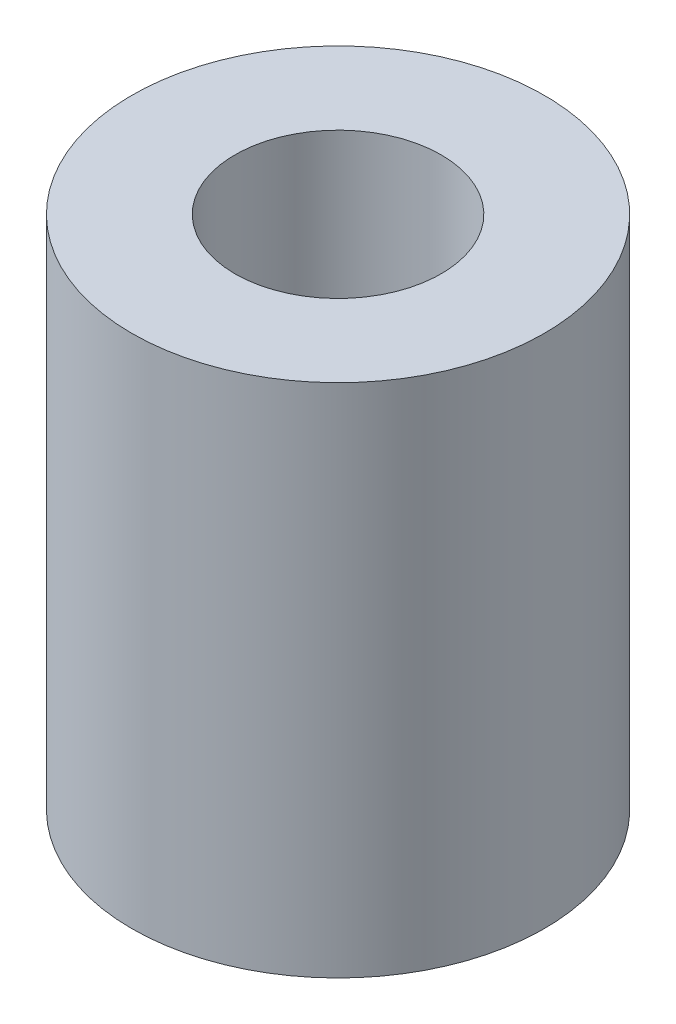
SolidWorks part; units mm, degrees
ref_plane "Front" through (0, 0, 0) normal (0, 0, 1) x (1, 0, 0)
ref_plane "Top" through (0, 0, 0) normal (0, 1, 0) x (1, 0, 0)
ref_plane "Right" through (0, 0, 0) normal (1, 0, 0) x (0, 0, -1)
sketch "Sketch1" plane through (0, 0, 0) normal (0, 1, 0) x (1, 0, 0)
  circle A0 centre (0, 0) radius 20
  circle A1 centre (0, 0) radius 10
  dimension "D1" = 40
  dimension "D2" = 20
extrude "Boss-Extrude1" add sketch "Sketch1" along normal blind 50
